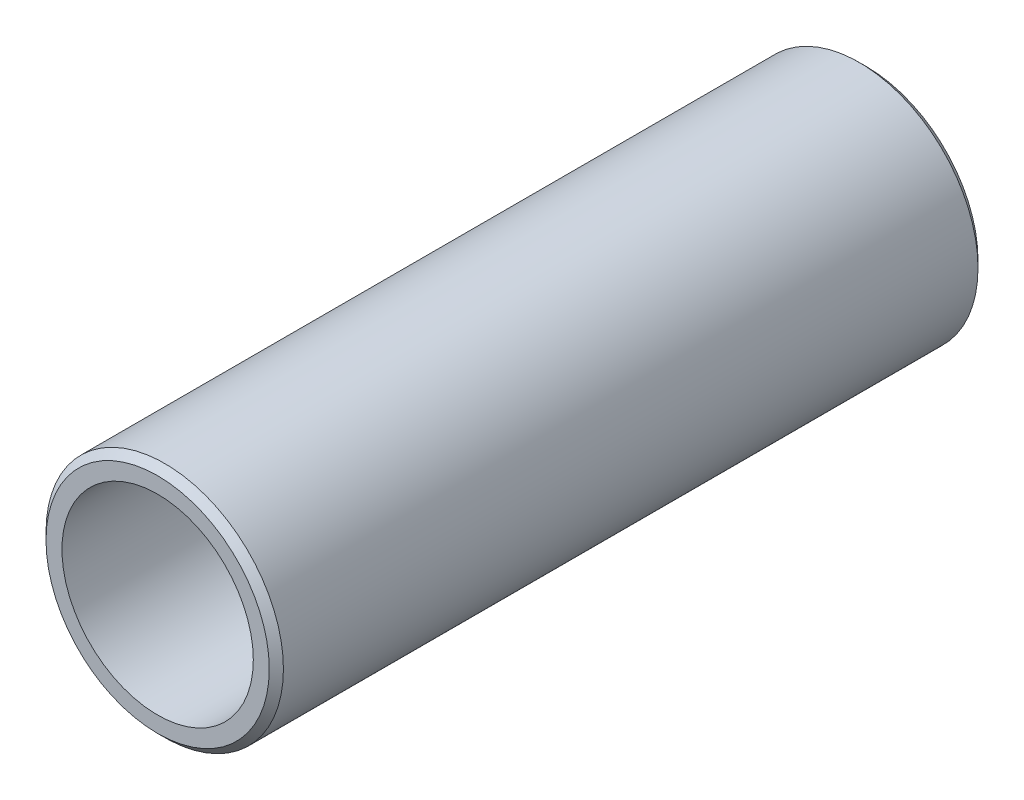
from build123d import *

# Parameters (mm, degrees)
SKETCH_1_R      = 16.75
SKETCH_1_R_2    = 13.5
EXTRUDE_1_DEPTH = 100
CHAMFER_1_SIZE  = 1
CHAMFER_2_SIZE  = 1


with BuildPart() as part:
    # 草图1 → 凸台-拉伸1 (new body)
    with BuildSketch(Plane.XY):
        Circle(SKETCH_1_R)
        Circle(SKETCH_1_R_2, mode=Mode.SUBTRACT)
    extrude(amount=EXTRUDE_1_DEPTH)

    # 倒角1
    chamfer_1_edges = [part.edges().sort_by_distance(p)[0] for p in [
        (-16.75, 0, 100),
    ]]
    chamfer(chamfer_1_edges, length=CHAMFER_1_SIZE)

    # 倒角2
    chamfer_2_edges = [part.edges().sort_by_distance(p)[0] for p in [
        (-16.75, 0, 0),
    ]]
    chamfer(chamfer_2_edges, length=CHAMFER_2_SIZE)


solid = part.part
